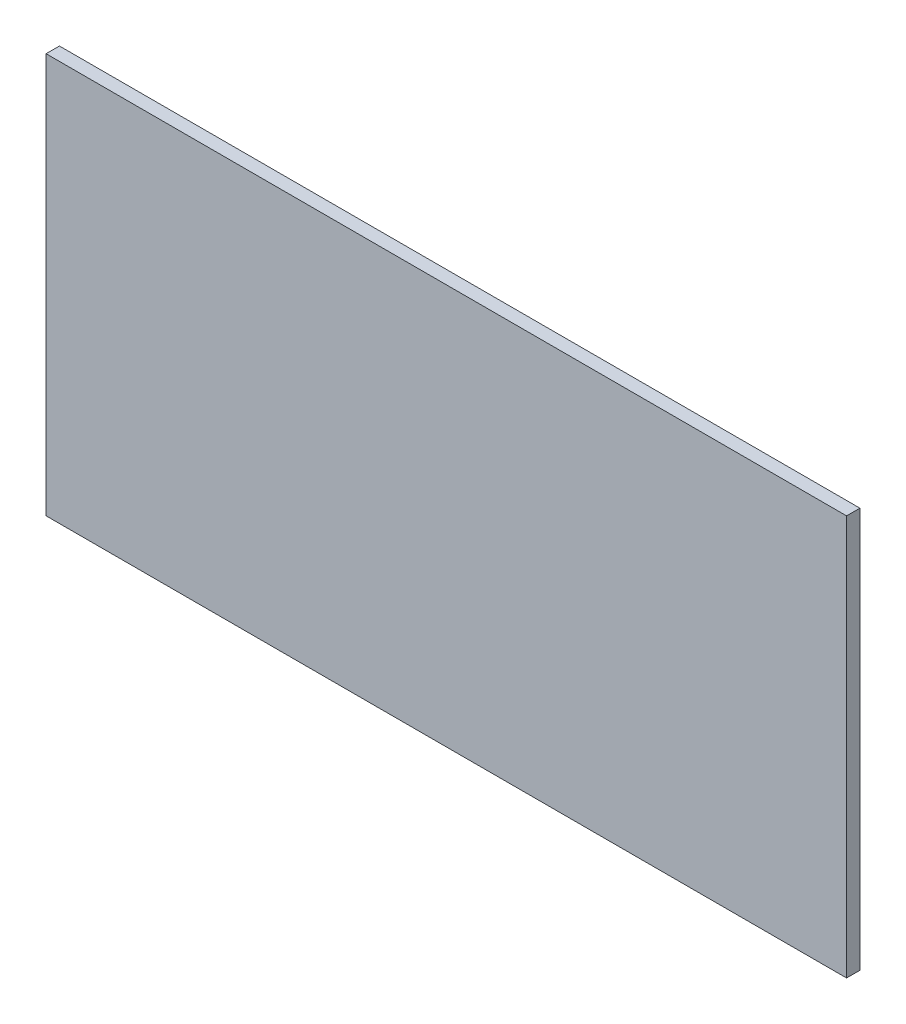
from build123d import *

# Parameters (mm, degrees)
SKETCH1_W           = 300
SKETCH1_H           = 150
BOSS_EXTRUDE1_DEPTH = 5


with BuildPart() as part:
    # Sketch1 → Boss-Extrude1 (new body)
    with BuildSketch(Plane.XY):
        with Locations((150, 75)):
            Rectangle(SKETCH1_W, SKETCH1_H)
    extrude(amount=BOSS_EXTRUDE1_DEPTH)


solid = part.part
